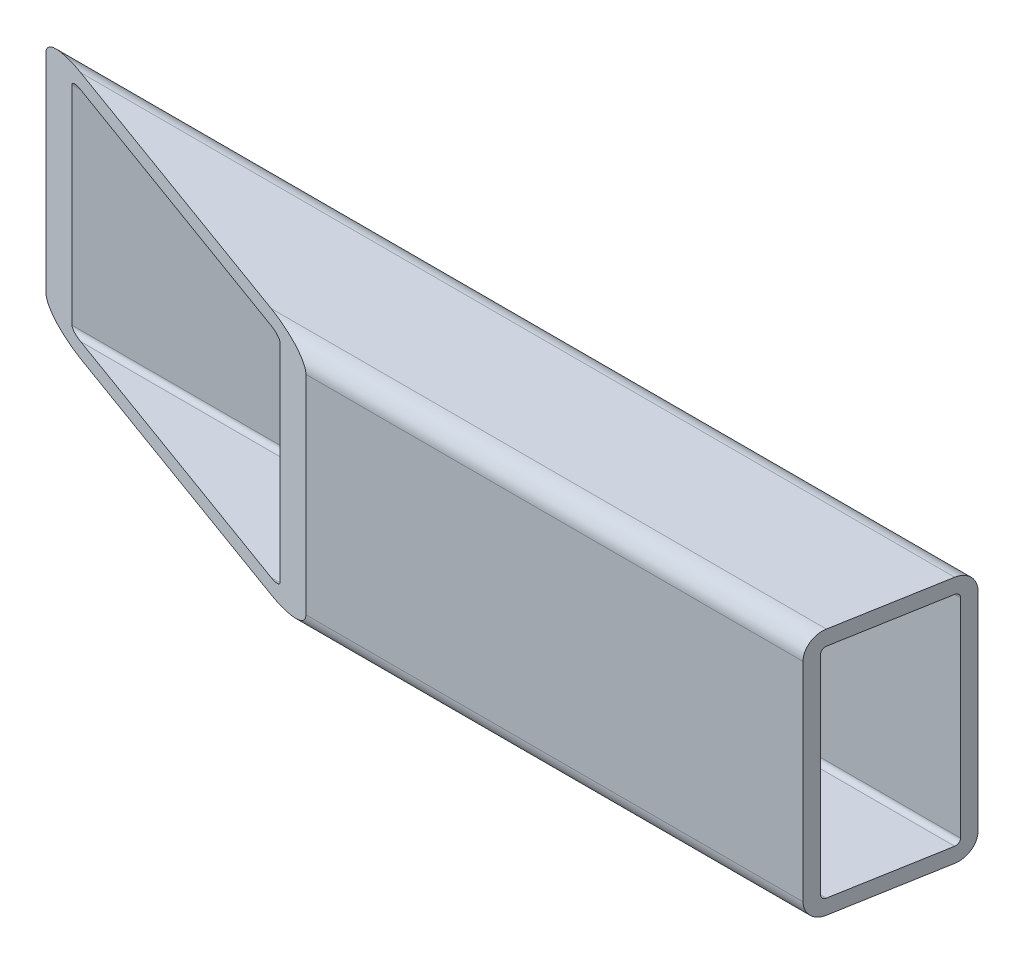
SolidWorks part; units mm, degrees
material "1023 碳钢板 (SS)"
ref_plane "Front Plane" through (0, 0, 0) normal (0, 0, 1) x (1, 0, 0)
ref_plane "Top Plane" through (0, 0, 0) normal (0, 1, 0) x (1, 0, 0)
ref_plane "Right Plane" through (0, 0, 0) normal (1, 0, 0) x (0, 0, -1)
sketch "草图1" plane through (0, 0, 0) normal (0, 0, 1) x (1, 0, 0)
  line L0 (0, 0) -> (200, 0)
  dimension "D1" = 200
other "Square tube 30 X 30 X 2.6(1)"
ref_plane "Plane1" through (0, 0, 0) normal (1, 0, 0) x (0, 1, 0)
sketch "Sketch1" plane through (0, 0, 0) normal (1, 0, 0) x (0, 1, 0)
  line L0 (-21, -12) -> (21, -12)
  line L1 (-22, -11) -> (-22, 11)
  line L2 (21, 12) -> (-21, 12)
  line L3 (22, 11) -> (22, -11)
  line L4 (-21, -15) -> (21, -15)
  line L5 (-25, -11) -> (-25, 11)
  line L6 (21, 15) -> (-21, 15)
  line L7 (25, 11) -> (25, -11)
  arc A0 (25, 11) -> (21, 15) centre (21, 11) ccw
  arc A1 (21, -15) -> (25, -11) centre (21, -11) ccw
  arc A2 (-25, -11) -> (-21, -15) centre (-21, -11) ccw
  arc A3 (-21, 15) -> (-25, 11) centre (-21, 11) ccw
  arc A4 (-21, 12) -> (-22, 11) centre (-21, 11) ccw
  arc A5 (22, 11) -> (21, 12) centre (21, 11) ccw
  arc A6 (21, -12) -> (22, -11) centre (21, -11) ccw
  arc A7 (-22, -11) -> (-21, -12) centre (-21, -11) ccw
  point P0 (-25, 0)
  point P1 (25, 0)
  point P2 (0, 15)
  point P3 (0, -15)
  point P4 (0, 0)
  point P5 (-25, -15)
  point P6 (25, -15)
  point P7 (25, 15)
  point P8 (-25, 15)
  point P33 (0, 0)
  dimension "D1" = 4
  dimension "D2" = 50
  dimension "Thickness" = 3
  dimension "V_leg" = 30
sketch "Sketch3" plane through (0, 25, 0) normal (0, 1, 0) x (1, 0, 0)
  line L0 (188, 15) -> (182.7102, -15)
  line L1 (200, 15) -> (0, 15) construction
  line L2 (200, -15) -> (0, -15) construction
  line L6 (188, 15) -> (200, 15)
  line L7 (200, 15) -> (200, -15)
  line L8 (200, -15) -> (182.7102, -15)
  dimension "D1" = 80
  dimension "D2" = 188
extrude "Cut-Extrude1" cut sketch "Sketch3" against normal blind 87
sketch "Sketch4" plane through (0, 25, 0) normal (0, 1, 0) x (1, 0, 0)
  line L0 (0, 15) -> (82.4243, -15)
  line L1 (182.7102, -15) -> (0, -15) construction
  line L2 (82.4243, -15) -> (0, -15)
  line L3 (0, -15) -> (0, 15)
  line L4 (188, 15) -> (0, 15) construction
  dimension "D1" = 20
extrude "Cut-Extrude2" cut sketch "Sketch4" against normal blind 137
